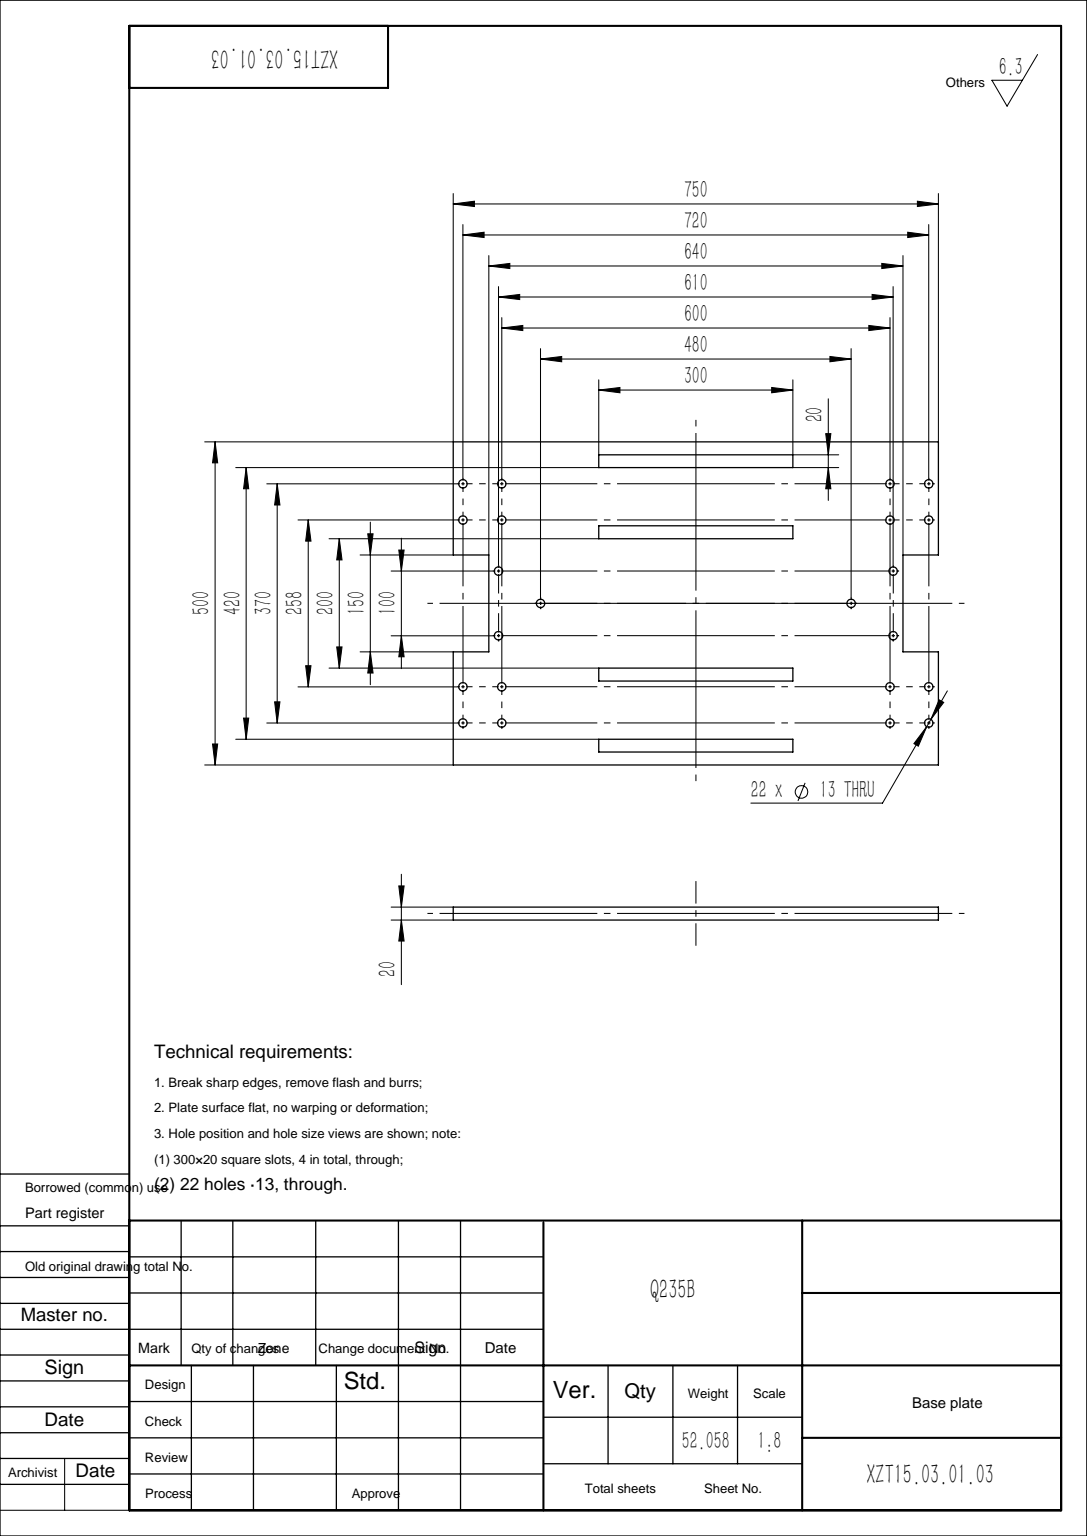
from build123d import *

# Parameters (mm, degrees)
SKETCH1_W                  = 300
SKETCH1_H                  = 20
BOSS_EXTRUDE1_DEPTH        = 20
F_13_0_13_DIAMETER_HOLE1_D = 13


with BuildPart() as part:
    # Sketch1 → Boss-Extrude1 (new body)
    with BuildSketch(Plane(origin=(0, 0, 0), x_dir=(1, 0, 0), z_dir=(0, 1, 0))):
        Polygon((-375, -250), (375, -250), (375, -75), (320, -75), (320, 75), (375, 75), (375, 250), (-375, 250), (-375, 75), (-320, 75), (-320, -75), (-375, -75), align=None)
        with Locations((0, -220)):
            Rectangle(SKETCH1_W, SKETCH1_H, mode=Mode.SUBTRACT)
        with Locations((0, -110)):
            Rectangle(SKETCH1_W, SKETCH1_H, mode=Mode.SUBTRACT)
        with Locations((0, 110)):
            Rectangle(SKETCH1_W, SKETCH1_H, mode=Mode.SUBTRACT)
        with Locations((0, 220)):
            Rectangle(SKETCH1_W, SKETCH1_H, mode=Mode.SUBTRACT)
    extrude(amount=BOSS_EXTRUDE1_DEPTH)

    # Ø13.0 (13) Diameter Hole1 (through all)
    with Locations(Plane(origin=(0, 20, 0), x_dir=(1, 0, 0), z_dir=(0, 1, 0))):
        with Locations((-360, 129), (-305, 50), (-240, 0), (-300, 129), (-300, 185), (-360, 185), (-360, -129), (-360, -185), (-300, -129), (-300, -185), (-305, -50), (360, -129), (300, -129), (360, -185), (360, 129), (360, 185), (300, 129), (305, -50), (300, -185), (300, 185), (240, 0), (305, 50)):
            Hole(F_13_0_13_DIAMETER_HOLE1_D / 2)


solid = part.part
